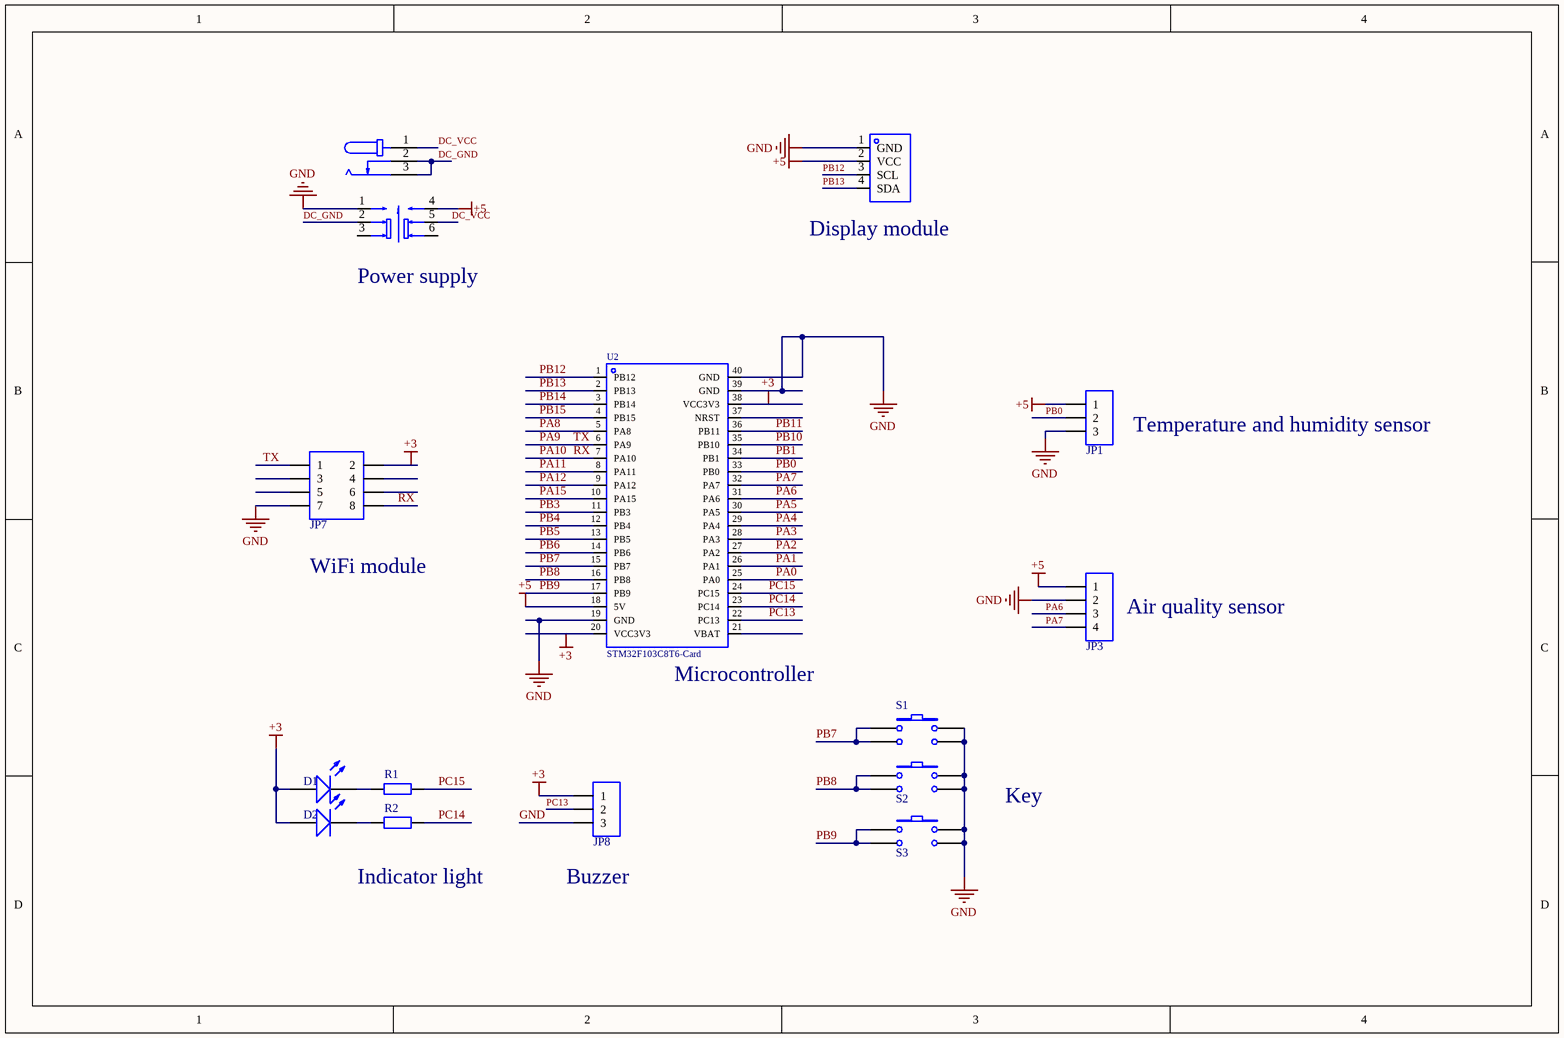
[diagram p0: MISC51894-3.schdoc]
# Altium project MISC51894-2.PrjPcb
1 sheet, 15 parts. Net scope: global (net labels, ports and power ports of the same name join across sheets).
Board file: MISC51894.pcbdoc

## Sheet MISC51894-3.schdoc
size 292 x 193 mm; SheetNumber: 1; SheetTotal: 1; Name: MISC51894

### Parts
D1  led  [LED-TH_5mm]  (value not drawn)
D2  led  [LED-TH_5mm]  (value not drawn)
DC1  DC002-1.3  [DC-IN-TH_DC002-1.3]  (value not drawn)
JP1  HDR-1X3  [HDR-TH_3P-P2.54-V-M-1]  (value not drawn)
JP3  HDR-1X4  [HDR-TH_4P-P2.54-V-M-1]  (value not drawn)
JP7  Header 4X2  [HDR-TH_8P-P2.54-V-F-R2-C4-S2.54-1]  (value not drawn)
JP8  HDR-1X3  [HDR-TH_3P-P2.54-V-M-1]  (value not drawn)
R1  Res2  [Res_1/8W]  (value not drawn)
R2  Res2  [Res_1/8W]  (value not drawn)
S1  key_4  [SW-TH_4P-L6.0-W6.0-P4.50-LS6.5]  (value not drawn)
S2  key_4  [SW-TH_4P-L6.0-W6.0-P4.50-LS6.5]  (value not drawn)
S3  key_4  [SW-TH_4P-L6.0-W6.0-P4.50-LS6.5]  (value not drawn)
SW1  Self-lock button  [SW-TH_6P-L7.0-W7.0-P2.00]  (value not drawn)
U1  OLED  [OLED-TH_L27.8-W27.2-P2.54_C9900033791]  (value not drawn)
U2  STM32F103C8T6-Card  [CONN-TH_L53.3-W22.9_STM32F103C8T6-CARD]

### Nets
+3: D1.1 D2.1 JP7.2 JP8.1 U2.20(VCC3V3) U2.38(VCC3V3)
+5: JP1.1 JP3.1 SW1.4 U1.2(VCC) U2.18(5V)
GND: JP1.3 JP3.2 JP7.7 JP8.3 S1.2 S1.4 S2.2 S2.4 S3.2 S3.4 SW1.1 U1.1(GND) U2.19(GND) U2.39(GND) U2.40(GND)
DC_GND: DC1.2 DC1.3 SW1.2
DC_VCC: DC1.1 SW1.5
PA0: U2.25(PA0)
PA1: U2.26(PA1)
PA2: U2.27(PA2)
PA3: U2.28(PA3)
PA4: U2.29(PA4)
PA5: U2.30(PA5)
PA6: JP3.3 U2.31(PA6)
PA7: JP3.4 U2.32(PA7)
PA8: U2.5(PA8)
PA9: JP7.1 U2.6(PA9)  [also labelled TX]
PA10: JP7.8 U2.7(PA10)  [also labelled RX]
PA11: U2.8(PA11)
PA12: U2.9(PA12)
PA15: U2.10(PA15)
PB0: JP1.2 U2.33(PB0)
PB1: U2.34(PB1)
PB3: U2.11(PB3)
PB4: U2.12(PB4)
PB5: U2.13(PB5)
PB6: U2.14(PB6)
PB7: S1.1 S1.3 U2.15(PB7)
PB8: S2.1 S2.3 U2.16(PB8)
PB9: S3.1 S3.3 U2.17(PB9)
PB10: U2.35(PB10)
PB11: U2.36(PB11)
PB12: U1.3(SCL) U2.1(PB12)
PB13: U1.4(SDA) U2.2(PB13)
PB14: U2.3(PB14)
PB15: U2.4(PB15)
PC13: JP8.2 U2.22(PC13)
PC14: R2.2 U2.23(PC14)
PC15: R1.2 U2.24(PC15)
NetD1_2: D1.2 R1.1
NetD2_2: D2.2 R2.1

Not connected (* = marked no-connect by the designer): JP7 3 4 5 6; SW1 3 6; U2 21(VBAT) 37(NRST)

### Notes on the sheet
- (near U1) Display module
- (near SW1) Power supply
- (near JP1) Temperature and humidity sensor
- (near JP7) WiFi module
- (near JP3) Air quality sensor
- (near U2) Microcontroller
- Key
- Indicator light
- (near JP8) Buzzer

### Library data of the parts
D1 = led: UniqueId: 6eb2f7ba7a12821c; AddInBom: yes; Device: led; Origin Footprint: led; DesignItemID: led; LibraryName: Schlib1; SymbolName: led
D2 = led: UniqueId: cca08e5caf06c018; AddInBom: yes; Device: led; Origin Footprint: led; DesignItemID: led; LibraryName: Schlib1; SymbolName: led
DC1 = DC002-1.3: Manufacturer: SHOU HAN(首韩); Add into BOM: yes; Connector Type: DC power socket; Inside Contact Diameter: 1.3mm; Outside Contact Diameter: 4.2mm; Current Rating (Max): 500mA; Voltage Rating (Max): 30V; UniqueId: 613237169519c5c2; ModelId: ccf1f99d79ab40ba9aeff26c21c7d5f10819f05c4eef4c71ace90d822a990e87; Device: DC002-1.3; LCSC Part Name: DC电源插座 内径:1.3mm 外径:4.2mm; Supplier Part: C668593; Manufacturer Part: DC002-1.3; Supplier Footprint: 插件; JLCPCB Part Class: Extended Part; Datasheet: https://atta.szlcsc.com/upload/public/pdf/source/20200619/C668593_6B5785499F122503841AA69BD23A954B.pdf; Supplier: LCSC; Convert to PCB: yes; Mounting Style: Right angle; Operating Temperature Range: -; Origin Footprint: DC-IN-TH_DC002-1.3; DesignItemID: DC002-1.3; LibraryName: Schlib1; SymbolName: DC002-1.3; FootprintName: DC-IN-TH_DC002-1.3; ModelName: DC-IN-TH_DC002-1.3
JP1 = Header 3: 3P connector; 学习资源: 最新版本发布; Origin Footprint: HDR2.54-LI-3P; UniqueId: 4fe8deccf3ecd12b; AddInBom: yes; Device: Header 3; BOM名称: 3P connector; DesignItemID: Header 3; LibraryName: 5.4 - Connector - pitch 2.54 (100mil); SymbolName: Header 3
JP3 = Header 4: 4P connector; 学习资源: 最新版本发布; Origin Footprint: HDR2.54-LI-4P; UniqueId: 4577e3d3da87c365; AddInBom: yes; Device: Header 4; BOM名称: 4P connector; DesignItemID: Header 4; LibraryName: 5.4 - Connector - pitch 2.54 (100mil); SymbolName: Header 4
JP7 = Header 4X2: 4*2P connector; Origin Footprint: HDR2.54-LI-2x4P; UniqueId: 2c2198ed19c983b6; AddInBom: yes; Device: Header 4X2; BOM名称: 4*2P connector; DesignItemID: Header 4X2; LibraryName: 5.4 - Connector - pitch 2.54 (100mil); SymbolName: Header 4X2
JP8 = Header 3: 3P connector; 学习资源: 最新版本发布; Origin Footprint: HDR2.54-LI-3P; UniqueId: 8401f236ce86758e; AddInBom: yes; Device: Header 3; BOM名称: 3P connector; DesignItemID: Header 3; LibraryName: 5.4 - Connector - pitch 2.54 (100mil); SymbolName: Header 3
R1 = Res2: Resistor; Origin Footprint: AXIAL0.4-1/4W; UniqueId: 353b166cc2dee846; AddInBom: yes; Device: Res2; Published: 8-Jun-2000; LatestRevisionDate: 17-Jul-2002; LatestRevisionNote: Re-released for DXP Platform.; PackageReference: AXIAL-0.4; DesignItemID: Res2; LibraryName: Miscellaneous Devices; SymbolName: Res2; Publisher: Altium Limited
R2 = Res2: Resistor; Origin Footprint: AXIAL0.4-1/4W; UniqueId: 6f63fc6711cfa315; AddInBom: yes; Device: Res2; Published: 8-Jun-2000; LatestRevisionDate: 17-Jul-2002; LatestRevisionNote: Re-released for DXP Platform.; PackageReference: AXIAL-0.4; DesignItemID: Res2; LibraryName: Miscellaneous Devices; SymbolName: Res2; Publisher: Altium Limited
S1 = key_4: UniqueId: 0ac0bd892f9b1ec0; AddInBom: yes; Device: key_4; Origin Footprint: key_4; DesignItemID: key_4; LibraryName: Schlib1; SymbolName: key_4
S2 = key_4: UniqueId: 16ca49f37df57620; AddInBom: yes; Device: key_4; Origin Footprint: key_4; DesignItemID: key_4; LibraryName: Schlib1; SymbolName: key_4
S3 = key_4: UniqueId: b21ed8cc1c3b642b; AddInBom: yes; Device: key_4; Origin Footprint: key_4; DesignItemID: key_4; LibraryName: Schlib1; SymbolName: key_4
SW1 = XKB7070-Z: Manufacturer: XKB Connectivity(中国星坤); Add into BOM: yes; Actuator Style: Rectangular button; Contact Current: 100mA; Voltage Rating (AC): 250V; Voltage Rating (DC): 30V; Insulation Resistance: 100MΩ; Actuator/Cap Color: Blue; With Lamp: Without; Pin Style: PC pin; Operating Force: 160gf; Mechanical Life: 10万 cycles; UniqueId: c39dab7994ba8bcb; ModelId: 65f5674ceb7247f197b01bc7adea0d8f0819f05c4eef4c71ace90d822a990e87; Device: XKB7070-Z; LCSC Part Name: 按键开关   7*7插件自锁 蓝白黑; Supplier Part: C318863; Manufacturer Part: XKB7070-Z; Supplier Footprint: 插件; JLCPCB Part Class: Extended Part; Datasheet: https://atta.szlcsc.com/upload/public/pdf/source/20211015/75A682A27A424BDE8D93C2CFA14C38FE.pdf; Supplier: LCSC; Convert to PCB: yes; Self Lock / No Lock: Self-lock; IP Rating: -; Mounting Style: Straight through-hole; Operating Temperature: -15℃~+55℃; Origin Footprint: SW-TH_6P-L7.0-W7.0-P2.00; DesignItemID: XKB7070-Z; LibraryName: Schlib1; SymbolName: XKB7070-Z; FootprintName: SW-TH_6P-L7.0-W7.0-P2.00; ModelName: SW-TH_6P-L7.0-W7.0-P2.00
U1 = OLED0.96: Manufacturer: HS(汉昇); Manufacturer Part: HS96L03W2C03; Add into BOM: yes; Main Control Chip: SSD1315; Interface Type: I2C; Pixel Resolution: 128x64; UniqueId: 1bdc0ab44f99f92d; ModelId: bb65183306db4ca69fb52250be49b00e0819f05c4eef4c71ace90d822a990e87; Device: OLED0.96; LCSC Part Name: 0.96寸OLED显示屏窄白光IIC; Supplier Part: C5248080; Supplier Footprint: -; JLCPCB Part Class: Extended Part; Datasheet: https://atta.szlcsc.com/upload/public/pdf/source/20230627/763D01F79A90007632F098068C7C8AD9.pdf; Supplier: LCSC; Convert to PCB: yes; Size: 0.96; Operating Temperature: -40℃~+70℃; Origin Footprint: OLED-TH_L27.8-W27.2-P2.54_C9900033791; DesignItemID: OLED0.96; LibraryName: Schlib1; SymbolName: OLED0.96; FootprintName: OLED-TH_L27.8-W27.2-P2.54_C9900033791; ModelName: OLED-TH_L27.8-W27.2-P2.54_C9900033791
U2 = STM32F103C8T6-Card: AddInBom: yes; ModelId: 70cdd142a616427fa7f75b03dcb285590819f05c4eef4c71ace90d822a990e87; ModelTransform: 2310.042,898.9982,0,0,0,0,90.551,0,-236.22; Symbol: STM32F103C8T6-CARD; Device: STM32F103C8T6-Card; LCSC Part Name: STM32F103C8T6-Card; SupplierPart: C9900077949; ManufacturerPart: STM32F103C8T6-Card; Supplier Footprint: 插件; JLCPCB Part Class: Extended Part; Supplier: LCSC; ConvertToPcb: yes; FootprintName: CONN-TH_L53.3-W22.9_STM32F103C8T6-CARD; ModelName: CONN-TH_L53.3-W22.9_STM32F103C8T6-CARD